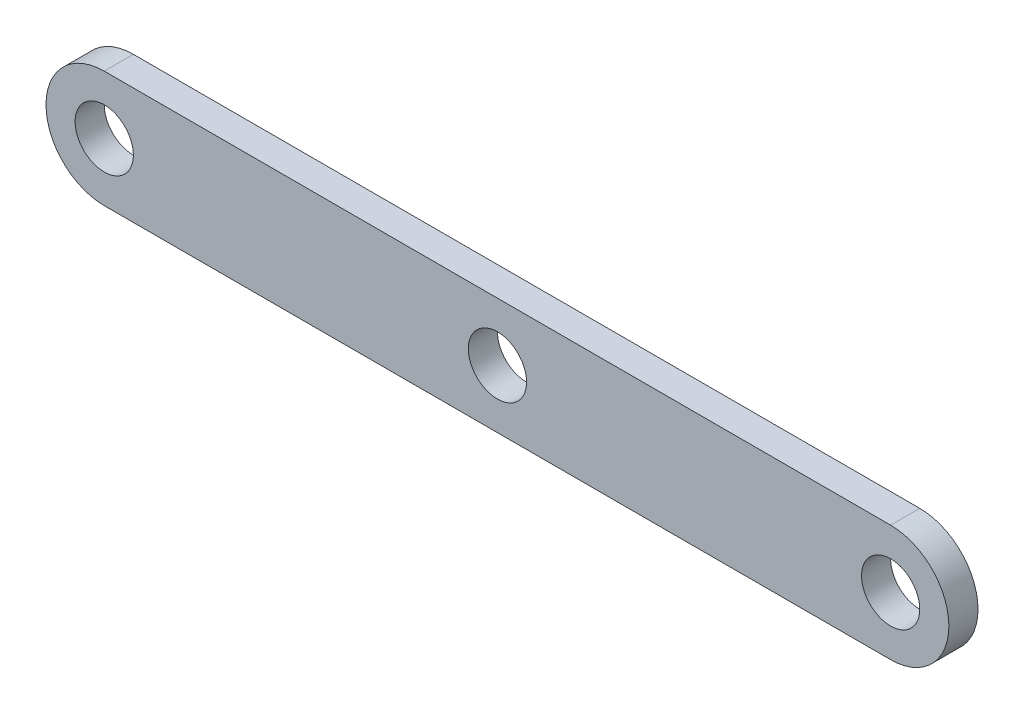
from build123d import *

# Parameters (mm, degrees)
BOSS_EXTRUDE1_DEPTH = 10
SKETCH2_R           = 10
CUT_EXTRUDE1_DEPTH  = 157.604597634
SKETCH3_R           = 10
CUT_EXTRUDE2_DEPTH  = 10


with BuildPart() as part:
    # Sketch1 → Boss-Extrude1 (new body)
    with BuildSketch(Plane.XY):
        with BuildLine():
            Line((-135, 20), (135, 20))
            ThreePointArc((135, 20), (155, 0), (135, -20))
            Line((135, -20), (-135, -20))
            ThreePointArc((-135, -20), (-155, 0), (-135, 20))
        make_face()
    extrude(amount=BOSS_EXTRUDE1_DEPTH)

    # Sketch2 → Cut-Extrude1 (cut, through all)
    with BuildSketch(Plane.XY.offset(10)):
        with Locations((-135, 0)):
            Circle(SKETCH2_R)
        with Locations((135, 0)):
            Circle(SKETCH2_R)
    extrude(amount=-CUT_EXTRUDE1_DEPTH, mode=Mode.SUBTRACT)

    # Sketch3 → Cut-Extrude2 (cut)
    with BuildSketch(Plane.XY.offset(10)):
        Circle(SKETCH3_R)
    extrude(amount=-CUT_EXTRUDE2_DEPTH, mode=Mode.SUBTRACT)


solid = part.part
